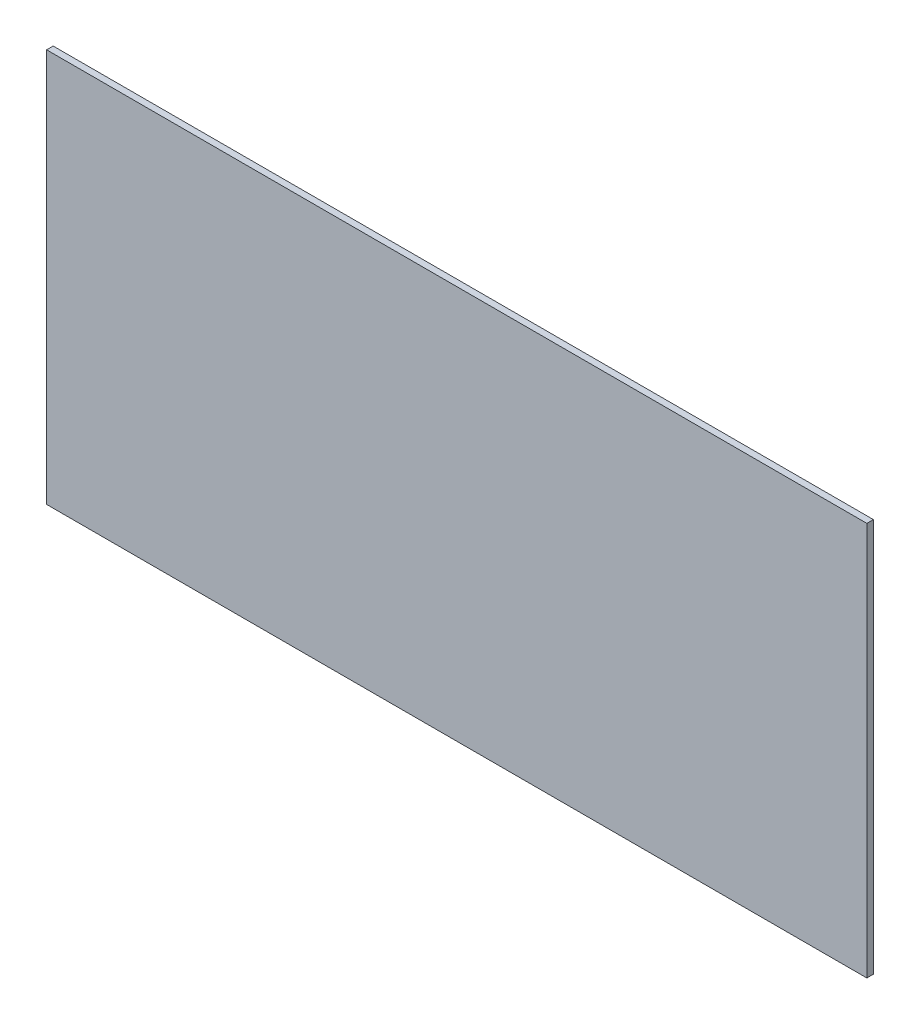
SolidWorks part; units mm, degrees
ref_plane "Front Plane" through (0, 0, 0) normal (0, 0, 1) x (1, 0, 0)
ref_plane "Top Plane" through (0, 0, 0) normal (0, 1, 0) x (1, 0, 0)
ref_plane "Right Plane" through (0, 0, 0) normal (1, 0, 0) x (0, 0, -1)
sketch "Sketch1" plane through (0, 0, 0) normal (0, 0, 1) x (1, 0, 0)
  line L1 (0, 0) -> (250, 0)
  line L2 (0, 0) -> (0, 120)
  line L3 (0, 120) -> (250, 120)
  line L4 (250, 0) -> (250, 120)
  dimension "D1" = 120
  dimension "D2" = 250
extrude "Boss-Extrude1" add sketch "Sketch1" along normal blind 2
